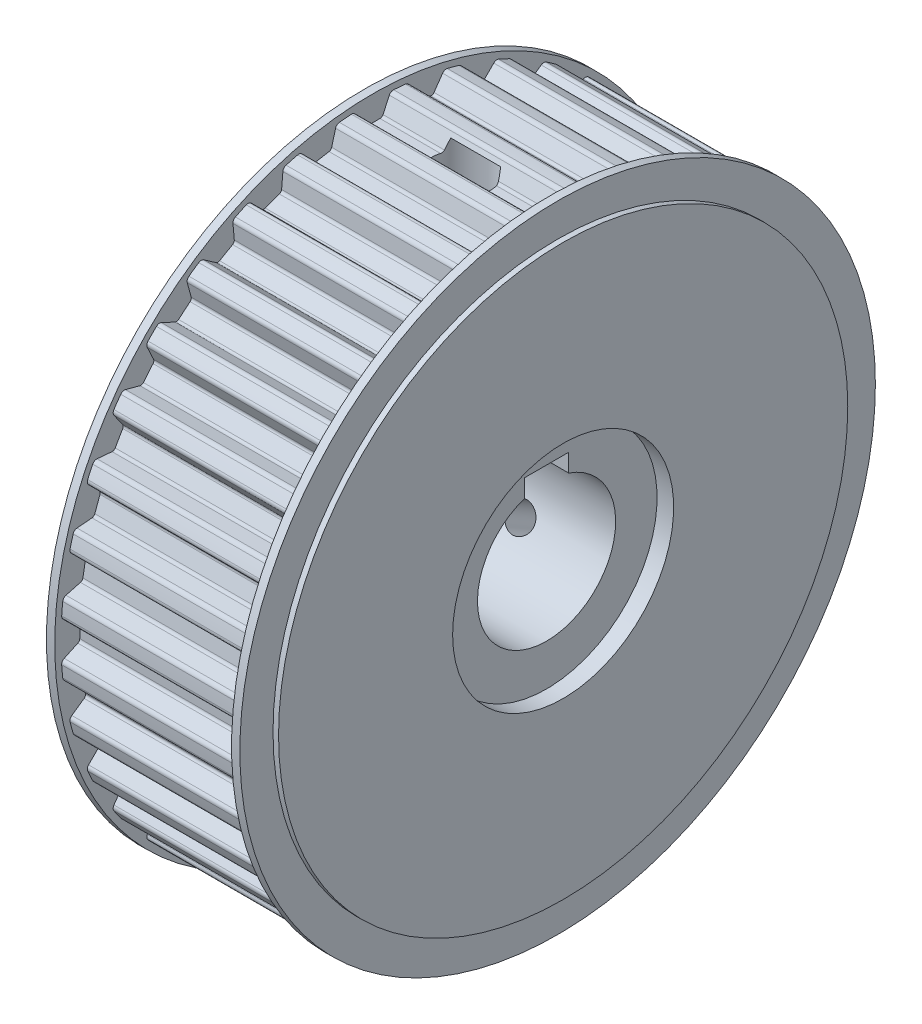
from build123d import *

# Parameters (mm, degrees)
SKETCH_1_R                       = 56.37
EXTRUDE_1_DEPTH                  = 16
CUT_EXTRUDE_2_DEPTH              = 32
FILLET_1_R                       = 0.6
FILLET_2_R                       = 0.8
PATTERN_CIRCULAR_1_COUNT         = 36
FILLET_1_OF_PATTERN_CIRCULAR_1_R = 0.6
FILLET_2_OF_PATTERN_CIRCULAR_1_R = 0.8
SKETCH_6_R                       = 57.5
EXTRUDE_2_DEPTH                  = 1.5
SKETCH_7_R                       = 51.5
EXTRUDE_3_DEPTH                  = 1
SKETCH_8_R                       = 12.5
CUT_EXTRUDE_1_DEPTH              = 90.339241098
SKETCH_11_R                      = 20
CUT_EXTRUDE_3_DEPTH              = 3
SKETCH_12_W                      = 8
SKETCH_12_H                      = 9.692858801
CUT_EXTRUDE_4_DEPTH              = 90.339241098
SKETCH_15_R                      = 5.25
CUT_EXTRUDE_5_DEPTH              = 22.76
PATTERN_CIRCULAR_2_COUNT         = 2
PATTERN_CIRCULAR_2_ANGLE         = 120


with BuildPart() as part:
    # 草图1 → 拉伸1 (new, symmetric)
    with BuildSketch(Plane(origin=(0, 0, 0), x_dir=(0, 0, -1), z_dir=(1, 0, 0))):
        Circle(SKETCH_1_R)
    extrude(amount=EXTRUDE_1_DEPTH, both=True)

    # 草图2 → Cut-Extrude 2 (cut)
    with BuildSketch(Plane(origin=(16, 0, 0), x_dir=(0, 0, -1), z_dir=(1, 0, 0))):
        with BuildLine():
            Line((-3.285, 56.274200794), (-1.744225866, 52.97))
            Line((-1.744225866, 52.97), (1.744225866, 52.97))
            Line((1.744225866, 52.97), (3.285, 56.274200794))
            ThreePointArc((3.285, 56.274200794), (0, 56.37), (-3.285, 56.274200794))
        make_face()
    cut_extrude_2 = extrude(amount=-CUT_EXTRUDE_2_DEPTH, mode=Mode.SUBTRACT)

    # 圆角1
    fillet_1_edges = [part.edges().sort_by_distance(p)[0] for p in [
        (0, 52.97, 1.744225866),
        (0, 52.97, -1.744225866),
    ]]
    fillet(fillet_1_edges, radius=FILLET_1_R)

    # 圆角2
    fillet_2_edges = [part.edges().sort_by_distance(p)[0] for p in [
        (0, 56.274200794, 3.285),
        (0, 56.274200794, -3.285),
    ]]
    fillet(fillet_2_edges, radius=FILLET_2_R)

    # 阵列(圆周)1: Cut-Extrude 2 ×36 about axis
    pattern_circular_1_axis = Axis((0, 0, 0), (1, 0, 0))
    for i in range(1, PATTERN_CIRCULAR_1_COUNT):
        add(cut_extrude_2.rotate(pattern_circular_1_axis, i * 360 / PATTERN_CIRCULAR_1_COUNT), mode=Mode.SUBTRACT)

    # 圆角1 of 阵列(圆周)1
    fillet_1_of_pattern_circular_1_edges = [part.edges().sort_by_distance(p)[0] for p in [
        (0, 51.862385034, 10.915871127),
        (0, 52.46814832, 7.480416815),
        (0, 49.178957742, 19.755843167),
        (0, 50.372078504, 16.477770817),
        (0, 45.001252706, 27.99554391),
        (0, 46.745478571, 24.97445609),
        (0, 39.456207377, 35.384614217),
        (0, 41.698540927, 32.712305153),
        (0, 32.712305153, 41.698540927),
        (0, 35.384614217, 39.456207377),
        (0, 24.97445609, 46.745478571),
        (0, 27.99554391, 45.001252706),
        (0, 16.477770817, 50.372078504),
        (0, 19.755843167, 49.178957742),
        (0, 7.480416815, 52.46814832),
        (0, 10.915871127, 51.862385034),
        (0, -1.744225866, 52.97),
        (0, 1.744225866, 52.97),
        (0, -10.915871127, 51.862385034),
        (0, -7.480416815, 52.46814832),
        (0, -19.755843167, 49.178957742),
        (0, -16.477770817, 50.372078504),
        (0, -27.99554391, 45.001252706),
        (0, -24.97445609, 46.745478571),
        (0, -35.384614217, 39.456207377),
        (0, -32.712305153, 41.698540927),
        (0, -41.698540927, 32.712305153),
        (0, -39.456207377, 35.384614217),
        (0, -46.745478571, 24.97445609),
        (0, -45.001252706, 27.99554391),
        (0, -50.372078504, 16.477770817),
        (0, -49.178957742, 19.755843167),
        (0, -52.46814832, 7.480416815),
        (0, -51.862385034, 10.915871127),
        (0, -52.97, -1.744225866),
        (0, -52.97, 1.744225866),
        (0, -51.862385034, -10.915871127),
        (0, -52.46814832, -7.480416815),
        (0, -49.178957742, -19.755843167),
        (0, -50.372078504, -16.477770817),
        (0, -45.001252706, -27.99554391),
        (0, -46.745478571, -24.97445609),
        (0, -39.456207377, -35.384614217),
        (0, -41.698540927, -32.712305153),
        (0, -32.712305153, -41.698540927),
        (0, -35.384614217, -39.456207377),
        (0, -24.97445609, -46.745478571),
        (0, -27.99554391, -45.001252706),
        (0, -16.477770817, -50.372078504),
        (0, -19.755843167, -49.178957742),
        (0, -7.480416815, -52.46814832),
        (0, -10.915871127, -51.862385034),
        (0, 1.744225866, -52.97),
        (0, -1.744225866, -52.97),
        (0, 10.915871127, -51.862385034),
        (0, 7.480416815, -52.46814832),
        (0, 19.755843167, -49.178957742),
        (0, 16.477770817, -50.372078504),
        (0, 27.99554391, -45.001252706),
        (0, 24.97445609, -46.745478571),
        (0, 35.384614217, -39.456207377),
        (0, 32.712305153, -41.698540927),
        (0, 41.698540927, -32.712305153),
        (0, 39.456207377, -35.384614217),
        (0, 46.745478571, -24.97445609),
        (0, 45.001252706, -27.99554391),
        (0, 50.372078504, -16.477770817),
        (0, 49.178957742, -19.755843167),
        (0, 52.46814832, -7.480416815),
        (0, 51.862385034, -10.915871127),
    ]]
    fillet(fillet_1_of_pattern_circular_1_edges, radius=FILLET_1_OF_PATTERN_CIRCULAR_1_R)

    # 圆角2 of 阵列(圆周)1
    fillet_2_of_pattern_circular_1_edges = [part.edges().sort_by_distance(p)[0] for p in [
        (0, 54.848834973, 13.007005886),
        (0, 55.9897035, 6.536818949),
        (0, 51.756915056, 22.33380048),
        (0, 54.003987398, 16.160019962),
        (0, 47.092387465, 30.981993848),
        (0, 50.377387465, 25.292206946),
        (0, 40.996981511, 38.688815011),
        (0, 45.220096107, 33.65590302),
        (0, 33.65590302, 45.220096107),
        (0, 38.688815011, 40.996981511),
        (0, 25.292206946, 50.377387465),
        (0, 30.981993848, 47.092387465),
        (0, 16.160019962, 54.003987398),
        (0, 22.33380048, 51.756915056),
        (0, 6.536818949, 55.9897035),
        (0, 13.007005886, 54.848834973),
        (0, -3.285, 56.274200794),
        (0, 3.285, 56.274200794),
        (0, -13.007005886, 54.848834973),
        (0, -6.536818949, 55.9897035),
        (0, -22.33380048, 51.756915056),
        (0, -16.160019962, 54.003987398),
        (0, -30.981993848, 47.092387465),
        (0, -25.292206946, 50.377387465),
        (0, -38.688815011, 40.996981511),
        (0, -33.65590302, 45.220096107),
        (0, -45.220096107, 33.65590302),
        (0, -40.996981511, 38.688815011),
        (0, -50.377387465, 25.292206946),
        (0, -47.092387465, 30.981993848),
        (0, -54.003987398, 16.160019962),
        (0, -51.756915056, 22.33380048),
        (0, -55.9897035, 6.536818949),
        (0, -54.848834973, 13.007005886),
        (0, -56.274200794, -3.285),
        (0, -56.274200794, 3.285),
        (0, -54.848834973, -13.007005886),
        (0, -55.9897035, -6.536818949),
        (0, -51.756915056, -22.33380048),
        (0, -54.003987398, -16.160019962),
        (0, -47.092387465, -30.981993848),
        (0, -50.377387465, -25.292206946),
        (0, -40.996981511, -38.688815011),
        (0, -45.220096107, -33.65590302),
        (0, -33.65590302, -45.220096107),
        (0, -38.688815011, -40.996981511),
        (0, -25.292206946, -50.377387465),
        (0, -30.981993848, -47.092387465),
        (0, -16.160019962, -54.003987398),
        (0, -22.33380048, -51.756915056),
        (0, -6.536818949, -55.9897035),
        (0, -13.007005886, -54.848834973),
        (0, 3.285, -56.274200794),
        (0, -3.285, -56.274200794),
        (0, 13.007005886, -54.848834973),
        (0, 6.536818949, -55.9897035),
        (0, 22.33380048, -51.756915056),
        (0, 16.160019962, -54.003987398),
        (0, 30.981993848, -47.092387465),
        (0, 25.292206946, -50.377387465),
        (0, 38.688815011, -40.996981511),
        (0, 33.65590302, -45.220096107),
        (0, 45.220096107, -33.65590302),
        (0, 40.996981511, -38.688815011),
        (0, 50.377387465, -25.292206946),
        (0, 47.092387465, -30.981993848),
        (0, 54.003987398, -16.160019962),
        (0, 51.756915056, -22.33380048),
        (0, 55.9897035, -6.536818949),
        (0, 54.848834973, -13.007005886),
    ]]
    fillet(fillet_2_of_pattern_circular_1_edges, radius=FILLET_2_OF_PATTERN_CIRCULAR_1_R)

    # 草图6 → 凸台-拉伸2 (add)
    with BuildSketch(Plane(origin=(16, 0, 0), x_dir=(0, 0, -1), z_dir=(1, 0, 0))):
        Circle(SKETCH_6_R)
    extrude_2 = extrude(amount=EXTRUDE_2_DEPTH)

    # 草图7 → 凸台-拉伸3 (add)
    with BuildSketch(Plane(origin=(17.5, 0, 0), x_dir=(0, 0, -1), z_dir=(1, 0, 0))):
        Circle(SKETCH_7_R)
    extrude_3 = extrude(amount=EXTRUDE_3_DEPTH)

    # 镜向2: 凸台-拉伸2, 凸台-拉伸3 across plane
    add(extrude_2.mirror(Plane(origin=(0, 0, 0), x_dir=(0, 0, 1), z_dir=(1, 0, 0))))
    add(extrude_3.mirror(Plane(origin=(0, 0, 0), x_dir=(0, 0, 1), z_dir=(1, 0, 0))))

    # 草图8 → 切除-拉伸1 (cut, through all)
    with BuildSketch(Plane.ZY.offset(18.5)):
        Circle(SKETCH_8_R)
    extrude(amount=-CUT_EXTRUDE_1_DEPTH, mode=Mode.SUBTRACT)

    # 草图11 → 切除-拉伸3 (cut)
    with BuildSketch(Plane.ZY.offset(18.5)):
        Circle(SKETCH_11_R)
    cut_extrude_3 = extrude(amount=-CUT_EXTRUDE_3_DEPTH, mode=Mode.SUBTRACT)

    # 镜向3: 切除-拉伸3 across plane
    add(cut_extrude_3.mirror(Plane(origin=(0, 0, 0), x_dir=(0, 0, 1), z_dir=(1, 0, 0))), mode=Mode.SUBTRACT)

    # 草图12 → 切除-拉伸4 (cut, through all)
    with BuildSketch(Plane.ZY.offset(18.5)):
        with Locations((0, 10.2535706)):
            Rectangle(SKETCH_12_W, SKETCH_12_H)
    extrude(amount=-CUT_EXTRUDE_4_DEPTH, mode=Mode.SUBTRACT)

    # 草图13 → M6 螺纹孔1 (revolve, cut)
    with BuildSketch(Plane(origin=(0, 55, 0), x_dir=(0, 0, 1), z_dir=(1, 0, 0))):
        Polygon((0, 0), (0, 51.502151548), (2.5, 50), (2.5, 0), align=None)
    hole_wizard_m6_1 = revolve(axis=Axis((0, 61.35, 0), (0, -1, 0)), mode=Mode.SUBTRACT)

    # 草图15 → 切除-拉伸5 (cut)
    with BuildSketch(Plane(origin=(0, 55, 0), x_dir=(1, 0, 0), z_dir=(0, 1, 0))):
        with Locations(Location((0, 0, 0), (0, 0, 270))):
            Circle(SKETCH_15_R)
    cut_extrude_5 = extrude(amount=-CUT_EXTRUDE_5_DEPTH, mode=Mode.SUBTRACT)

    # 阵列(圆周)2: M6 螺纹孔1, 切除-拉伸5 ×2 about axis
    pattern_circular_2_axis = Axis((18.5, 0, 0), (-1, 0, 0))
    add([hole_wizard_m6_1.rotate(pattern_circular_2_axis, i * PATTERN_CIRCULAR_2_ANGLE / (PATTERN_CIRCULAR_2_COUNT - 1)) for i in range(1, PATTERN_CIRCULAR_2_COUNT)], mode=Mode.SUBTRACT)
    add([cut_extrude_5.rotate(pattern_circular_2_axis, i * PATTERN_CIRCULAR_2_ANGLE / (PATTERN_CIRCULAR_2_COUNT - 1)) for i in range(1, PATTERN_CIRCULAR_2_COUNT)], mode=Mode.SUBTRACT)


solid = part.part
